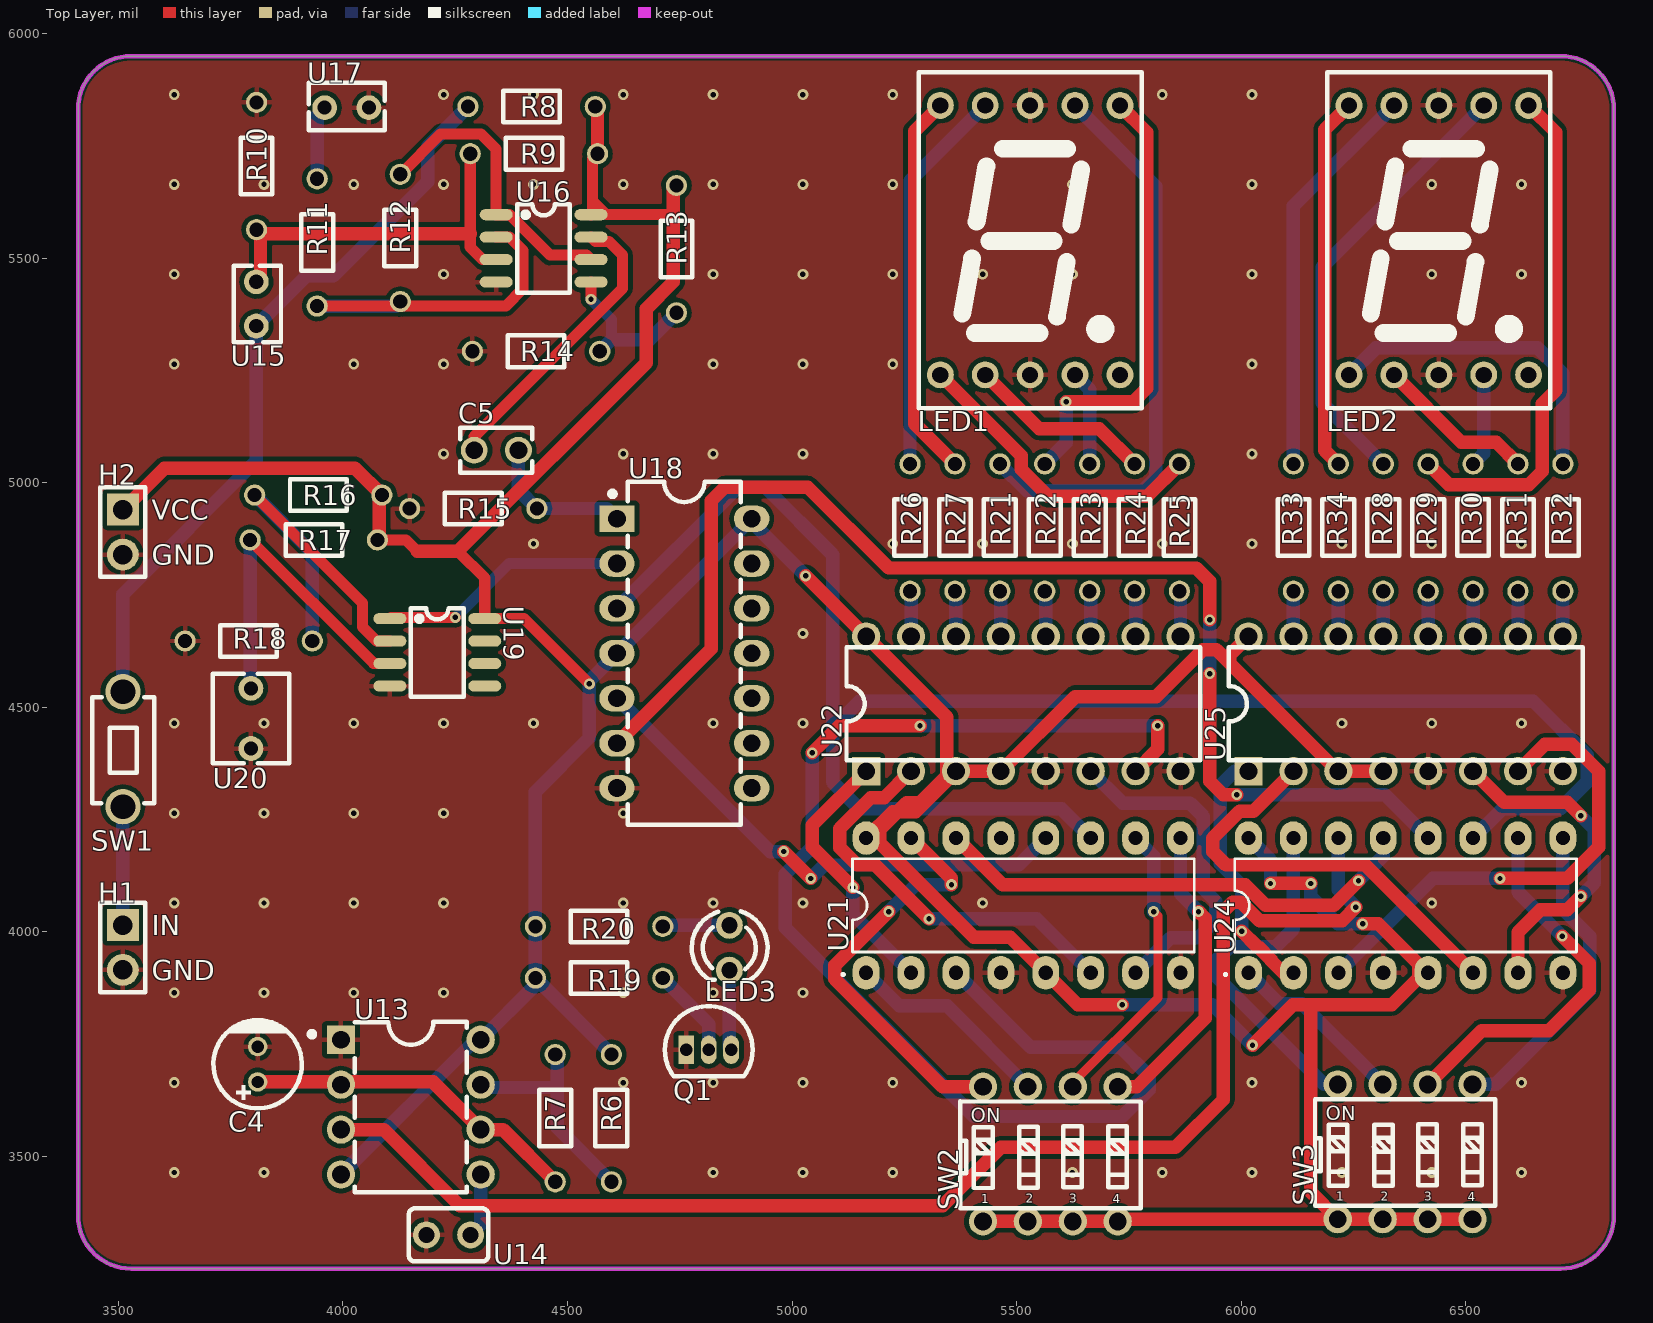
[diagram p0: Top Layer view]
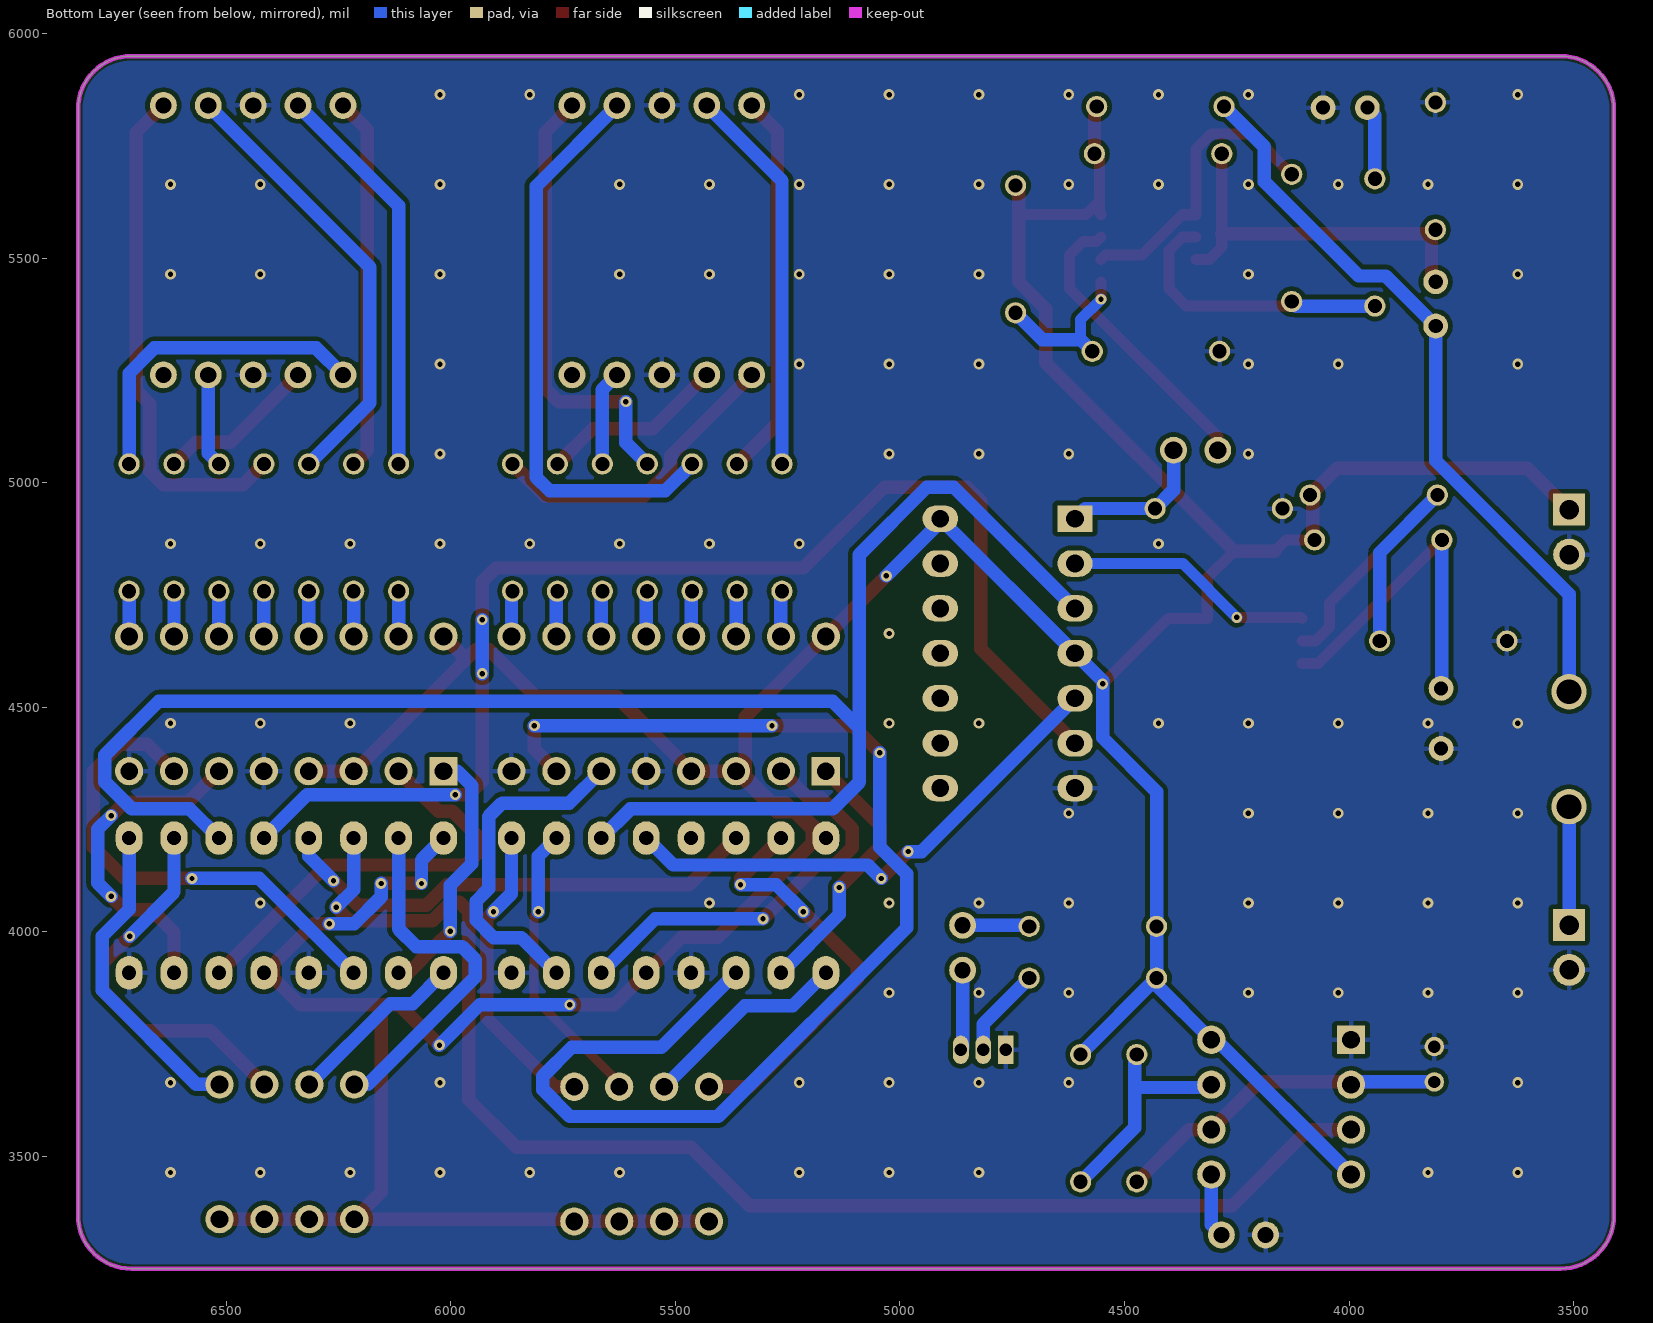
[diagram p1: Bottom Layer view, seen from below]
# Altium PCB MISC51104.pcbdoc
Units mil, origin at the board's own origin, x right, y up, seen from the top; angles counter-clockwise.
Board outline 3420 x 2700 mil, 2 copper layers (Top Layer, Bottom Layer), stack 62.206 mil thick; 52 components, 69 nets, 219 pads, 135 vias.

## Layer stack, top to bottom
Top Solder Mask Layer: solder mask 0.394, Dk 3.3
Top Layer: signal copper 1.379
Dielectric1: surface 59.449, FR4, Dk 4.5
Bottom Layer: signal copper 1.378
Bottom Solder Mask Layer: solder mask 0.394, Dk 3.3

## Board outline
3528.11,5950 ccw(c3528.11,5831.89) 3410,5831.89 3410,3368.11 ccw(c3528.11,3368.11) 3528.11,3250 6711.89,3250 ccw(c6711.89,3368.11) 6830,3368.11 6830,5831.89 ccw(c6711.89,5831.89) 6711.89,5950

## Design rules (kind name [scope] priority, off if disabled: settings)
BoardOutlineClearance copperThickness2oz_1 [All] p2 off: genericclearance=7.99 ignorepadtopadclearanceinfootprint=FALSE except(0: Arc-SplitContinuation Track-SplitContinuation SMDPad-SplitContinuation THPad-SplitContinuation Via-SplitContinuation Fill-SplitContinuation Region-SplitContinuation Poly-SplitContinuation Text-SplitContinuation Hole-SplitContinuation; 5.98: Arc-CutoutEdge Track-CutoutEdge SMDPad-CutoutEdge THPad-CutoutEdge Via-CutoutEdge Text-CutoutEdge; 6.89: Hole-OutlineEdge Hole-CutoutEdge; 10: Poly-OutlineEdge Poly-CutoutEdge; 11.81: Arc-OutlineEdge Track-OutlineEdge SMDPad-OutlineEdge THPad-OutlineEdge Via-OutlineEdge Fill-OutlineEdge Region-OutlineEdge Text-OutlineEdge Fill-CutoutEdge Region-CutoutEdge)
BoardOutlineClearance Plane_innerPlane_1 [All] p4 off: genericclearance=4.02 ignorepadtopadclearanceinfootprint=FALSE except(0: Arc-SplitContinuation Track-SplitContinuation SMDPad-SplitContinuation THPad-SplitContinuation Via-SplitContinuation Fill-SplitContinuation Region-SplitContinuation Poly-SplitContinuation Text-SplitContinuation Hole-SplitContinuation; 5.98: Arc-CutoutEdge Track-CutoutEdge SMDPad-CutoutEdge THPad-CutoutEdge Via-CutoutEdge Text-CutoutEdge; 6.89: Hole-OutlineEdge Hole-CutoutEdge; 10: Poly-OutlineEdge Poly-CutoutEdge; 11.81: Arc-OutlineEdge Track-OutlineEdge SMDPad-OutlineEdge THPad-OutlineEdge Via-OutlineEdge Fill-OutlineEdge Region-OutlineEdge Text-OutlineEdge Fill-CutoutEdge Region-CutoutEdge)
BoardOutlineClearance Copper_copperRegion_1 [All] p6 off: genericclearance=4.02 ignorepadtopadclearanceinfootprint=FALSE except(0: Arc-SplitContinuation Track-SplitContinuation SMDPad-SplitContinuation THPad-SplitContinuation Via-SplitContinuation Fill-SplitContinuation Region-SplitContinuation Poly-SplitContinuation Text-SplitContinuation Hole-SplitContinuation; 5.98: Arc-CutoutEdge Track-CutoutEdge SMDPad-CutoutEdge THPad-CutoutEdge Via-CutoutEdge Text-CutoutEdge; 6.89: Hole-OutlineEdge Hole-CutoutEdge; 10: Poly-OutlineEdge Poly-CutoutEdge; 11.81: Arc-OutlineEdge Track-OutlineEdge SMDPad-OutlineEdge THPad-OutlineEdge Via-OutlineEdge Fill-OutlineEdge Region-OutlineEdge Text-OutlineEdge Fill-CutoutEdge Region-CutoutEdge)
BoardOutlineClearance copperThickness1oz_1 [All] p8: genericclearance=4.02 ignorepadtopadclearanceinfootprint=FALSE except(0: Arc-SplitContinuation Track-SplitContinuation SMDPad-SplitContinuation THPad-SplitContinuation Via-SplitContinuation Fill-SplitContinuation Region-SplitContinuation Poly-SplitContinuation Text-SplitContinuation Hole-SplitContinuation; 5.98: Arc-CutoutEdge Track-CutoutEdge SMDPad-CutoutEdge THPad-CutoutEdge Via-CutoutEdge Text-CutoutEdge; 6.89: Hole-OutlineEdge Hole-CutoutEdge; 10: Poly-OutlineEdge Poly-CutoutEdge; 11.81: Arc-OutlineEdge Track-OutlineEdge SMDPad-OutlineEdge THPad-OutlineEdge Via-OutlineEdge Fill-OutlineEdge Region-OutlineEdge Text-OutlineEdge Fill-CutoutEdge Region-CutoutEdge)
Clearance copperThickness2oz [All] p1 off: gap=7.99 ignorepadtopadclearanceinfootprint=FALSE except(5.98: SMDPad-Track SMDPad-SMDPad THPad-Track SMDPad-THPad THPad-THPad Track-Via SMDPad-Via THPad-Via Via-Via Fill-SMDPad Region-SMDPad Fill-THPad Region-THPad Fill-Via Region-Via Fill-Fill Fill-Region Region-Region Arc-Track Arc-SMDPad Arc-THPad Arc-Via Fill-Arc Region-Arc Arc-Arc Text-Track SMDPad-Text Text-THPad Text-Via Fill-Text Region-Text Arc-Text Text-Text; 6.89: Hole-Track Hole-SMDPad Hole-THPad Hole-Via Fill-Hole Region-Hole Hole-Arc Hole-Text; 10: Poly-Track Poly-SMDPad Poly-THPad Poly-Via Poly-Fill Poly-Region Poly-Poly Poly-Arc Poly-Text Poly-Hole; 11.81: Fill-Track Region-Track)
Clearance Plane_innerPlane [All] p3 off: gap=4.02 ignorepadtopadclearanceinfootprint=FALSE except(5.98: SMDPad-Track SMDPad-SMDPad THPad-Track SMDPad-THPad THPad-THPad Track-Via SMDPad-Via THPad-Via Via-Via Fill-SMDPad Region-SMDPad Fill-THPad Region-THPad Fill-Via Region-Via Fill-Fill Fill-Region Region-Region Arc-Track Arc-SMDPad Arc-THPad Arc-Via Fill-Arc Region-Arc Arc-Arc Text-Track SMDPad-Text Text-THPad Text-Via Fill-Text Region-Text Arc-Text Text-Text; 6.89: Hole-Track Hole-SMDPad Hole-THPad Hole-Via Fill-Hole Region-Hole Hole-Arc Hole-Text; 10: Poly-Track Poly-SMDPad Poly-THPad Poly-Via Poly-Fill Poly-Region Poly-Poly Poly-Arc Poly-Text Poly-Hole; 11.81: Fill-Track Region-Track)
Clearance Copper_copperRegion [All] p5 off: gap=4.02 ignorepadtopadclearanceinfootprint=FALSE except(5.98: SMDPad-Track SMDPad-SMDPad THPad-Track SMDPad-THPad THPad-THPad Track-Via SMDPad-Via THPad-Via Via-Via Fill-SMDPad Region-SMDPad Fill-THPad Region-THPad Fill-Via Region-Via Fill-Fill Fill-Region Region-Region Arc-Track Arc-SMDPad Arc-THPad Arc-Via Fill-Arc Region-Arc Arc-Arc Text-Track SMDPad-Text Text-THPad Text-Via Fill-Text Region-Text Arc-Text Text-Text; 6.89: Hole-Track Hole-SMDPad Hole-THPad Hole-Via Fill-Hole Region-Hole Hole-Arc Hole-Text; 10: Poly-Track Poly-SMDPad Poly-THPad Poly-Via Poly-Fill Poly-Region Poly-Poly Poly-Arc Poly-Text Poly-Hole; 11.81: Fill-Track Region-Track)
Clearance copperThickness1oz [All] p7: gap=4.02 ignorepadtopadclearanceinfootprint=FALSE except(5.98: SMDPad-Track SMDPad-SMDPad THPad-Track SMDPad-THPad THPad-THPad Track-Via SMDPad-Via THPad-Via Via-Via Fill-SMDPad Region-SMDPad Fill-THPad Region-THPad Fill-Via Region-Via Fill-Fill Fill-Region Region-Region Arc-Track Arc-SMDPad Arc-THPad Arc-Via Fill-Arc Region-Arc Arc-Arc Text-Track SMDPad-Text Text-THPad Text-Via Fill-Text Region-Text Arc-Text Text-Text; 6.89: Hole-Track Hole-SMDPad Hole-THPad Hole-Via Fill-Hole Region-Hole Hole-Arc Hole-Text; 10: Poly-Track Poly-SMDPad Poly-THPad Poly-Via Poly-Fill Poly-Region Poly-Poly Poly-Arc Poly-Text Poly-Hole; 11.81: Fill-Track Region-Track)
DiffPairsRouting differentialPair [All] p1: maxlimit=6 minlimit=6 mostfreqgap=6 toplayer_minwidth=5 toplayer_prefwidth=10 toplayer_maxwidth=100 toplayer_mingap=6 toplayer_prefgap=6 toplayer_maxgap=6 bottomlayer_minwidth=5 bottomlayer_prefwidth=10 bottomlayer_maxwidth=100 bottomlayer_mingap=6 bottomlayer_prefgap=6 bottomlayer_maxgap=6 maxuncoupledlength=10
HoleToHoleClearance otherClearance [All] p1: gap=11.81 allowstackedmicrovias=TRUE
Length netLength [All] p1: minlimit=0 maxlimit=0
PasteMaskExpansion pasteMaskExpansion [All] p1: expansion=0
PlaneConnect innerPlane [All] p1: planeconnectstyle=Relief reliefexpansion=20 reliefentries=4 reliefconductorwidth=10 reliefairgap=10
PolygonConnect copperRegion [All] p1: connectstyle=Relief reliefconductorwidth=10 reliefentries=4 polygonreliefangle="90 Angle" airgapwidth=10 via.connectstyle=Relief via.reliefconductorwidth=10 via.reliefentries=4 via.polygonreliefangle="90 Angle" via.airgapwidth=10
RoutingVias viaSize [All] p1: holewidth=12.01 width=24.02 viastyle="Through Hole" minholewidth=11.81 minwidth=19.68 maxholewidth=248.03 maxwidth=393.7
SolderMaskExpansion solderMaskExpansion [IsVia] p1: expansion=-1000 istentingtop=TRUE
SolderMaskExpansion solderMaskExpansion [All] p2: expansion=2.01 istentingtop=FALSE
Width copperThickness2oz_2 [All] p1 off: maxlimit=100 minlimit=8 preferedwidth=10
Width copperThickness1oz_2 [All] p2: maxlimit=100 minlimit=5 preferedwidth=30

## Components (designator, comment, footprint, x,y, rotation, side; value= is the part's Value field where it differs from the comment)
C4 "10uF" CAP-TH_BD5.0-P2.00-D0.5-FD 3810,3705 r90 top
C5 "100nF" CAP-TH_L4.0-W2.5-P2.50-D0.5-A 4341.4,5072.26 r0 top
H1 "" HDR-TH_2P-P2.54-V-M-1 3510,3965 r270 top
H2 "" HDR-TH_2P-P2.54-V-M-1 3510,4890 r270 top
LED1 "" LED-SEG-TH_10P-L12.6-W19.0-P2.54-S15.24-BL 5530,5540 r0 top
LED2 "" LED-SEG-TH_10P-L12.6-W19.0-P2.54-S15.24-BL 6440,5540 r0 top
LED3 "" LED_TH-3mm 4860.3,3964.43 r270 top
Q1 "2N2222A" TO-92-3_L4.9-W3.7-P1.27-L 4814.38,3737.18 r0 top
R6 "47kΩ" Res_1/8W 4600,3585 r90 top
R7 "47kΩ" Res_1/8W 4475,3585 r90 top
R8 "4.7kΩ" Res_1/8W 4420,5835 r0 top
R9 "4.7kΩ" Res_1/8W 4425,5730 r0 top
R10 "4.7kΩ" Res_1/8W 3805,5705 r270 top
R11 "1kΩ" Res_1/8W 3940,5535 r270 top
R12 "100kΩ" Res_1/8W 4130,5545 r90 top
R13 "10kΩ" Res_1/8W 4745,5520 r90 top
R14 "2kΩ" Res_1/8W 4430,5290 r0 top
R15 "10kΩ" Res_1/8W 4290,4940 r0 top
R16 "100kΩ" Res_1/8W 3945,4970 r0 top
R17 "100kΩ" Res_1/8W 3935,4870 r0 top
R18 "100kΩ" Res_1/8W 3790,4645 r0 top
R19 "3kΩ" Res_1/8W 4570.3,3899.43 r180 top
R20 "200Ω" Res_1/8W 4570.3,4014.43 r180 top
R21 "10kΩ" Res_1/8W 5465,4900 r90 top
R22 "10kΩ" Res_1/8W 5565,4900 r90 top
R23 "10kΩ" Res_1/8W 5665,4900 r90 top
R24 "10kΩ" Res_1/8W 5765,4900 r90 top
R25 "10kΩ" Res_1/8W 5865,4900 r90 top
R26 "10kΩ" Res_1/8W 5265,4900 r90 top
R27 "10kΩ" Res_1/8W 5365,4900 r90 top
R28 "10kΩ" Res_1/8W 6318.74,4900 r90 top
R29 "10kΩ" Res_1/8W 6418.74,4900 r90 top
R30 "10kΩ" Res_1/8W 6518.74,4900 r90 top
R31 "10kΩ" Res_1/8W 6618.74,4900 r90 top
R32 "10kΩ" Res_1/8W 6718.74,4900 r90 top
R33 "10kΩ" Res_1/8W 6118.74,4900 r90 top
R34 "10kΩ" Res_1/8W 6218.74,4900 r90 top
SW1 "" Key_TH_3.5x6x4.3 3510,4400 r90 top
SW2 "拨码开关EI-04" SW-TH_DIPSWITCHEI-04 5575,3505 r0 top
SW3 "拨码开关EI-04" SW-TH_DIPSWITCHEI-04 6365,3510 r0 top
U13 "NE555PE4" PDIP-8_L9.6-W6.4-P2.54-LS7.9-BL-1 4151.02,3609.58 r270 top
U14 "100nF" CAP-TH_L4.5-W3.0-P2.50-D0.5 4235,3325 r0 top
U15 "1uF" CAP-TH_L4.0-W2.5-P2.50-D0.5 3806.97,5398.05 r90 top
U16 "LM358AD" SOP-8_L4.9-W3.9-P1.27-LS6.0-BL 4446.68,5521.68 r270 top
U17 "1uF" CAP-TH_L4.0-W2.5-P2.50-D0.5 4008.42,5835 r180 top
U18 "CD4011BD" PDIP-14_L19.3-W6.4-P2.54-LS7.9-BL-1 4760,4620 r270 top
U19 "LM358AD" SOP-8_L4.9-W3.9-P1.27-LS6.0-BL 4210.07,4622.26 r270 top
U20 "光敏电阻-5MM" RES-TH_L4.9-W4.3-P3.4 3795,4475 r90 top
U21 "SN74LS190N" PDIP-16_L19.2-W6.6-P2.54-LS7.6-BL 5514.82,4058.71 r0 top
U22 "CD4511BE" DIP-16_L19.8-W6.5-P2.54-LS7.6-BL 5514.82,4507.64 r0 top
U24 "SN74LS190N" PDIP-16_L19.2-W6.6-P2.54-LS7.6-BL 6366.27,4058.71 r0 top
U25 "CD4511BE" DIP-16_L19.8-W6.5-P2.54-LS7.6-BL 6366.27,4507.64 r0 top

## Footprints (in the part's own frame and the unit in brackets; to place one, negate y for a bottom-side part, rotate by r counter-clockwise, add the part's x,y. Pads: shape width x height; smd on the part's side, far side on the other; paste and mask are expansions set on the pad)
CAP-TH_BD5.0-P2.00-D0.5-FD [mm]
  round 1.1 hole 0.7 paste+0 mask+0.05: 1(-1,0) 2(1,0)
  silkscreen extent -2.5,-2.5 2.5,2.5
CAP-TH_L4.0-W2.5-P2.50-D0.5 [mm]
  round 1.4 hole 0.8 paste+0 mask+0.05: 1(-1.25,0) 2(1.25,0)
  silkscreen extent -2.16,-1.4 2.16,1.27
CAP-TH_L4.0-W2.5-P2.50-D0.5-A [mil]
  round 60 hole 39.37 paste+0 mask+1.97: 1(-49.21,0) 2(49.21,0)
  silkscreen extent -80,-50 80,50
CAP-TH_L4.5-W3.0-P2.50-D0.5 [mil]
  round 60 hole 36 paste+0 mask+1.97: 1(-49.21,0) 2(49.21,0)
  silkscreen extent -89,-59 89,59
DIP-16_L19.8-W6.5-P2.54-LS7.6-BL [mm]
  rect 1.6x1.6 hole 1: 1(-8.89,-3.81)
  round 1.6 hole 1 copper offset 0,0: 2(-6.35,-3.81) 3(-3.81,-3.81) 4(-1.27,-3.81) 5(1.27,-3.81) 6(3.81,-3.81) 7(6.35,-3.81) 8(8.89,-3.81) 9(8.89,3.81) 10(6.35,3.81) 11(3.81,3.81) 12(1.27,3.81) 13(-1.27,3.81) 14(-3.81,3.81) 15(-6.35,3.81) 16(-8.89,3.81)
  silkscreen extent -10,-3.2 10,3.2
HDR-TH_2P-P2.54-V-M-1 [mm]
  rect 1.8x1.8 hole 1.1: 1(-1.27,0)
  round 1.8 hole 1.1: 2(1.27,0)
  silkscreen extent -2.54,-1.27 2.54,1.27
Key_TH_3.5x6x4.3 [mil]
  round 78.7 hole 55.1 paste+0 mask+2: A(-121.44,0) B(134.46,0)
  silkscreen extent -114,-70 123,68
LED-SEG-TH_10P-L12.6-W19.0-P2.54-S15.24-BL [mil]
  round 60 hole 36: 1(-200,-300) 2(-100,-300) 3(0,-300) 4(100,-300) 5(200,-300) 6(200,300) 7(100,300) 8(0,300) 9(-100,300) 10(-200,300)
  silkscreen extent -248,-374 248,374
LED_TH-3mm [mil]
  round 60 hole 36 paste+0 mask+2: 1(-50,0) 2(50,0)
  silkscreen extent -81,-84 72,85
PDIP-8_L9.6-W6.4-P2.54-LS7.9-BL-1 [mil]
  rect 63x63 hole 39.37: 1(-150,-155.51)
  round 63 hole 39.37: 2(-50,-155.51) 3(50,-155.51) 4(150,-155.51) 5(150,155.52) 6(50,155.52) 7(-50,155.52) 8(-150,155.52)
  silkscreen extent -190,-226 190,125
PDIP-14_L19.3-W6.4-P2.54-LS7.9-BL-1 [mm]
  rect 1.5x2 hole 1: 1(-7.62,-3.81)
  oval 1.5x2 hole 1: 2(-5.08,-3.81) 3(-2.54,-3.81) 4(0,-3.81) 5(2.54,-3.81) 6(5.08,-3.81) 7(7.62,-3.81)
  oval 1.5x2 hole 1 copper offset 0,0: 8(7.62,3.81) 9(5.08,3.81) 10(2.54,3.81) 11(0,3.81) 12(-2.54,3.81) 13(-5.08,3.81) 14(-7.62,3.81)
  silkscreen extent -9.7,-4.21 9.7,3.2
PDIP-16_L19.2-W6.6-P2.54-LS7.6-BL [mm]
  oval 1.52x1.9 hole 0.8: 1(-8.89,-3.81) 2(-6.35,-3.81) 3(-3.81,-3.81) 4(-1.27,-3.81) 5(1.27,-3.81) 6(3.81,-3.81) 7(6.35,-3.81) 8(8.89,-3.81) 9(8.89,3.81) 10(6.35,3.81) 11(3.81,3.81) 12(1.27,3.81) 13(-1.27,3.81) 14(-3.81,3.81) 15(-6.35,3.81) 16(-8.89,3.81)
  silkscreen extent -10.26,-3.98 9.66,2.63
RES-TH_L4.9-W4.3-P3.4 [mm]
  round 1.4 hole 0.8 paste+0 mask+0.05: 1(-1.7,0) 2(1.7,0)
  silkscreen extent -2.54,-2.16 2.54,2.16
Res_1/8W [mil]
  round 47.2 hole 31.5 paste+0 mask+2: 1(-141.7,2.48) 2(141.7,2.48)
  silkscreen extent -63,-33 63,38
SOP-8_L4.9-W3.9-P1.27-LS6.0-BL [mm]
  oval 0.63x1.865 smd: 1(-1.905,-2.682) 2(-0.635,-2.682) 3(0.635,-2.682) 4(1.905,-2.682) 5(1.905,2.682) 6(0.635,2.682) 7(-0.635,2.682) 8(-1.905,2.682)
  silkscreen extent -2.5,-1.5 2.5,1.48
SW-TH_DIPSWITCHEI-04 [mm]
  round 1.6 hole 1: 1(-3.81,-3.81) 2(-1.27,-3.81) 3(1.27,-3.81) 4(3.81,-3.81) 5(3.81,3.81) 6(1.27,3.81) 7(-1.27,3.81) 8(-3.81,3.81)
  silkscreen extent -5.1,-3.05 5.11,2.98
TO-92-3_L4.9-W3.7-P1.27-L [mm]
  rect 0.9x1.6 hole 0.7: 1(-1.27,0)
  oval 0.9x1.6 hole 0.7: 2(0,0) 3(1.27,0)
  silkscreen extent -2.48,-1.5 2.48,2.48

## Via types
v1: diameter 24.02, hole 12, Top Layer to Bottom Layer, 134 vias
v2: diameter 24, hole 12, Top Layer to Bottom Layer, 1 vias

## Nets (pads, with @x,y where several pads share a name; then routed paths per layer and width w, separated by ;. In a path a pad name is that pad's centre, name@x,y a point inside that pad or via, vN(x,y) a via of type N, cw(c..) or ccw(c..) an arc to the next point about the centre after c; other vN are vias at no path point)
$1N1893: R6.1 R7.2 U13.7 | length 508.8
  Bottom Layer w30: U13.7 4312.81,3653.3 4477.52,3653.3 ; R7.2 4477.52,3721.7 4477.52,3653.3 ; R6.1 4477.52,3563.3 4477.52,3653.3
$1N1894: C4.1 R7.1 U13.2 U13.6 | length 942.6
  Top Layer w30: C4.1 4200.48,3665.63 U13.6 4356.25,3559.58 R7.1
  Bottom Layer w30: C4.1 3989.46,3665.63 U13.2
$1N1895: U13.5 U14.2 | length 143.8
  Bottom Layer w30: U14.2 4306.53,3347.32 U13.5
$1N1964: H1.1 SW1.A | length 263.6
  Bottom Layer w30: H1.1 SW1.A
$1N2089: R8.1 SW1.B U15.1 | length 1656.4
  Bottom Layer w30: SW1.B 3510,4751.87 3806.97,5048.84 U15.1 3918.3,5460.17 3978.3,5460.17 4188.3,5670.17 4188.3,5747.48 R8.1
$1N2753: R9.1 R10.2 U15.2 U16.3 | length 867.9
  Top Layer w24.8: R9.1 4283.3,5554.44 4283.3,5524.44 4311.07,5496.68 U16.3
  Top Layer w30: U15.2 3816.33,5456.63 R10.2@3816.33,5554.44 ; R10.2 R10.2@3816.33,5554.44 ; 4283.3,5554.44 R10.2@3816.33,5554.44
$1N2866: R11.1 U17.2 | length 165.2
  Bottom Layer w30: R11.1 3942.48,5818.27 U17.2
$1N2941: R12.2 U16.1 U16.6 | length 663.8
  Top Layer w24.8: R12.2 4217.52,5776.7 4307.52,5776.7 4341.07,5743.16 U16.1 4371.07,5596.68 4461.07,5506.68 4542.29,5506.68 U16.6
$1N2947: R11.2 R12.1 U16.2 | length 821
  Top Layer w24.8: R11.2 4362.48,5393.3 4401.07,5431.89 4401.07,5516.68 4371.07,5546.68 U16.2
  Bottom Layer w30: R11.2 4117.52,5393.3 R12.1
$1N3011: R13.1 R14.2 U16.5 | length 353.5
  Top Layer w24.8: v1(4552.29,5408.3) U16.5
  Bottom Layer w24.8: v1(4552.29,5408.3) 4597.52,5363.06 4597.52,5318.3
  Bottom Layer w30: R14.2 4597.52,5318.3 4682.52,5318.3 R13.1
$1N3176: C5.1 U16.7 | length 657.6
  Top Layer w24.8: C5.1 4292.19,5102.26 4622.19,5432.26 4622.19,5506.77 4592.19,5536.77 4562.19,5536.77 U16.7
$1N3286: C5.2 R15.2 U18.1 | length 334.4
  Bottom Layer w30: C5.2 4390.61,4983.56 R15.2 4587.53,4942.48 U18.1
$1N6918: U18.2 U19.1 | length 556.4
  Top Layer w24.8: U19.1 4107.2,4700 v1(4250,4700)
  Bottom Layer w24.8: v1(4250,4700) 4370,4820 U18.2
$1N7003: R17.1 U19.3 U20.2 | length 756.4
  Top Layer w24.8: R17.1 4068.52,4597.26 U19.3
  Bottom Layer w30: R17.1 3793.3,4543.63 U20.2
$1N7096: R16.1 R18.2 U19.2 | length 845.7
  Top Layer w24.8: R16.1 4043.3,4732.48 4043.3,4678.42 4074.46,4647.26 U19.2
  Bottom Layer w30: R16.1 3931.7,4844.08 R18.2
$1N10184: R26.1 U22.15 | length 101.6
  Bottom Layer w30: R26.1 5264.82,4756.01 U22.15
$1N10187: LED1.9 R26.2 | length 867.7
  Bottom Layer w30: R26.2 5262.52,5672.52 LED1.9
$1N10190: R27.1 U22.14 | length 101.6
  Bottom Layer w30: R27.1 5364.82,4756.01 U22.14
$1N10193: LED1.10 R27.2 | length 859.4
  Top Layer w30: LED1.10 5272.52,5782.52 5272.52,5131.7 R27.2
$1N10196: R21.1 U22.13 | length 101.6
  Bottom Layer w30: R21.1 5464.82,4756.01 U22.13
$1N10199: LED1.7 R21.2 | length 1287.6
  Bottom Layer w30: R21.2 5522.52,4981.7 5780,4981.7 5810,5011.7 5810,5660 LED1.7
$1N10202: R22.1 U22.12 | length 101.6
  Bottom Layer w30: R22.1 5564.82,4756.01 U22.12
$1N10205: LED1.6 R22.2 | length 1005.2
  Top Layer w30: v1(5610,5180) 5760,5180 5790,5210 5790,5780 LED1.6
  Bottom Layer w30: R22.2 5610,5089.18 v1(5610,5180)
$1N10208: R23.1 U22.11 | length 101.6
  Bottom Layer w30: R23.1 5664.82,4756.01 U22.11
$1N10211: LED1.4 R23.2 | length 211.8
  Bottom Layer w30: LED1.4 5662.52,5207.48 R23.2
$1N10214: R24.1 U22.10 | length 101.6
  Bottom Layer w30: R24.1 5764.82,4756.01 U22.10
$1N10217: LED1.2 R24.2 | length 414.7
  Top Layer w30: LED1.2 5550,5120 5684.22,5120 R24.2
$1N10220: R25.1 U22.9 | length 101.6
  Bottom Layer w30: R25.1 5864.82,4756.01 U22.9
$1N10223: LED1.1 R25.2 | length 691.6
  Top Layer w30: LED1.1 5510,5060 5510,5030 5570,4970 5790.82,4970 R25.2
$1N10225: U21.2 U22.1 | length 589.8
  Top Layer w30: v1(5134.82,4098.71) 5044.82,4188.71 5044.82,4237.64 U22.1
  Bottom Layer w30: v1(5134.82,4098.71) 5134.82,4038.71 U21.2
$1N10227: U21.3 U22.7 | length 2894.1
  Top Layer w30: v1(5044.82,4398.71) 5104.82,4458.71 v1(5284.82,4458.71) ; U22.7 5813.75,4406.57 v1(5813.75,4458.71)
  Bottom Layer w30: v1(5044.82,4398.71) 5044.82,4188.71 4984.82,4128.71 4984.82,4008.71 5404.82,3588.71 5734.82,3588.71 5794.82,3648.71 5794.82,3678.71 5730.88,3742.64 5530.88,3742.64 U21.3 ; v1(5284.82,4458.71) v1(5813.75,4458.71)
$1N10229: U21.6 U22.2 | length 928.4
  Top Layer w30: U22.2 5263.75,4357.64 5204.82,4298.71 5174.82,4298.71 5106.03,4229.92 5106.03,4187.49 5144.82,4148.71 5184.82,4148.71 v1(5304.82,4028.71)
  Bottom Layer w30: v1(5304.82,4028.71) 5544.82,4028.71 U21.6
$1N10231: U21.7 U22.6 | length 762.7
  Bottom Layer w30: U22.6 5735.89,4286.57 5885.89,4286.57 5915.89,4256.57 5915.89,4095.5 5943.6,4067.78 5943.6,4025.35 5904.82,3986.57 5842.68,3986.57 U21.7
$1N10411: SW2.7 U21.1 | length 465.3
  Bottom Layer w30: U21.1 5238.52,3835 5345,3835 SW2.7
$1N10413: SW2.5 U21.9 | length 682.2
  Top Layer w30: SW2.5 5767.43,3655 5920,3807.57 5920,4030 v1(5905,4045)
  Bottom Layer w30: U21.9 5864.82,4085.18 v1(5905,4045)
$1N10415: SW2.6 U21.10 | length 653.2
  Top Layer w20: SW2.6 5625,3663.31 5815,3853.31 5815,4035 v1(5805,4045)
  Bottom Layer w30: U21.10 5805,4168.52 v1(5805,4045)
$1N10417: SW2.8 U21.15 | length 934.8
  Top Layer w30: v1(5215,4045) 5095,3925 5095,3895 5335,3655 SW2.8 ; U21.15 5354.82,4118.71 v1(5354.82,4105)
  Bottom Layer w30: v1(5215,4045) 5275,4105 v1(5354.82,4105)
$1N10829: U24.2 U25.1 | length 575.2
  Top Layer w30: v1(6001.27,4001.11) 6035.28,3967.09 6037.35,3967.09 6067.17,3937.27 6067.17,3935.2 6093.67,3908.71 U24.2
  Bottom Layer w30: v1(6001.27,4001.11) 6001.27,4103.71 5953.23,4151.74 5953.23,4325.67 5985.2,4357.64 U25.1
$1N10831: U24.6 U25.2 | length 963.5
  Top Layer w30: U25.2 6027.34,4268.71 5996.27,4268.71 5936.27,4208.71 5936.27,4178.71 5966.27,4148.71 6276.27,4148.71 U24.6
$1N10833: U24.7 U25.6 | length 749
  Top Layer w30: U25.6 6585.2,4288.71 6726.27,4288.71 v1(6756.27,4258.71) ; U24.7 6616.27,3998.71 6666.27,4048.71 6726.27,4048.71 v1(6756.27,4078.71)
  Bottom Layer w30: v1(6756.27,4078.71) 6786.27,4108.71 6786.27,4228.71 v1(6756.27,4258.71)
$1N10844: SW3.5 U24.9 | length 711.8
  Bottom Layer w30: SW3.5 6566.27,3660 6776.27,3870 6776.27,3990 6716.27,4050 U24.9
$1N10846: SW3.7 U24.1 | length 401.8
  Bottom Layer w30: U24.1 6084.97,3840 6135,3840 SW3.7
$1N10848: SW3.6 U24.10 | length 851.4
  Top Layer w30: SW3.6 6535,3780 6685,3780 6775,3870 6775,3930 v1(6715,3990)
  Bottom Layer w30: U24.10 6616.27,4088.73 v1(6715,3990)
$1N10850: LED2.6 R29.2 | length 1137.2
  Top Layer w30: R29.2 6462.53,4995.43 6640,4995.43 6670,5025.43 6670,5175.43 6700,5205.43 6700,5780 LED2.6
$1N10852: LED2.4 R30.2 | length 208.1
  Bottom Layer w30: R30.2 6540,5065.43 LED2.4
$1N10854: LED2.2 R31.2 | length 358.4
  Top Layer w30: LED2.2 6490,5090 6567.97,5090 R31.2
$1N10856: LED2.1 R32.2 | length 726.5
  Bottom Layer w30: LED2.1 6300,5300 6660,5300 6716.27,5243.73 R32.2
$1N10858: LED2.9 R33.2 | length 891
  Bottom Layer w30: R33.2 6116.27,5616.27 LED2.9
$1N10860: LED2.10 R34.2 | length 833
  Top Layer w30: R34.2 6186.27,5071.7 6186.27,5786.27 LED2.10
$1N10862: R33.1 U25.15 | length 100.7
  Bottom Layer w30: U25.15 R33.1
$1N10864: R34.1 U25.14 | length 100.7
  Bottom Layer w30: U25.14 R34.1
$1N10866: R29.1 U25.12 | length 100.7
  Bottom Layer w30: U25.12 R29.1
$1N10868: R30.1 U25.11 | length 100.7
  Bottom Layer w30: U25.11 R30.1
$1N10870: R31.1 U25.10 | length 100.7
  Bottom Layer w30: U25.10 R31.1
$1N10872: R32.1 U25.9 | length 100.7
  Bottom Layer w30: U25.9 R32.1
$1N10874: SW3.8 U24.15 | length 808.9
  Bottom Layer w30: U24.15 6116.27,4006.27 6077.09,3967.09 5975,3967.09 5945,3937.09 5945,3900 6185,3660 SW3.8
$1N10876: U24.3 U25.7 | length 1094.6
  Top Layer w30: v1(6576.27,4118.71) 6726.27,4118.71 6796.27,4188.71 6796.27,4357.64 6736.27,4417.64 6676.27,4417.64 U25.7
  Bottom Layer w30: U24.3 6426.27,4118.71 v1(6576.27,4118.71)
$1N10878: R28.1 U25.13 | length 100.7
  Bottom Layer w30: U25.13 R28.1
$1N10880: LED2.7 R28.2 | length 1003.9
  Bottom Layer w30: R28.2 6180,5177.97 6180,5480 LED2.7
$1N10977: U18.3 U21.11 U24.11 | length 3907
  Bottom Layer w30: U18.3 4880,4990 4940,4990 5090,4840 5090,4453.52 ; U21.11 5600,4273.52 5150,4273.52 5090,4333.52 5090,4453.52 ; U24.11 6581.08,4273.52 6710,4273.52 6770,4333.52 6770,4393.52 6650,4513.52 5150,4513.52 5090,4453.52
$1N10992: U21.14 U24.13 | length 1099.1
  Top Layer w30: U21.14 5468.52,4105 6008.52,4105 6054.82,4058.71 6206.27,4058.71 v1(6261.27,4113.71)
  Bottom Layer w30: v1(6261.27,4113.71) 6316.27,4168.71 U24.13
$1N11009: U18.5 U21.12 | length 1158.3
  Top Layer w30: v1(4981.29,4178.71) v1(5041.29,4118.71)
  Bottom Layer w30: U18.5 4951.29,4178.71 v1(4981.29,4178.71) ; v1(5041.29,4118.71) 5071.29,4148.71 5504.82,4148.71 U21.12
$1N11018: U18.6 U24.12 | length 2820
  Top Layer w30: U18.6 4820,4630 4820,4960 4850,4990 5035,4990 5215,4810 5900,4810 5930,4780 v1(5930,4694.97) ; v1(5930,4574.97) 5930,4334.97 5960,4304.97 v1(5990,4304.97)
  Bottom Layer w30: v1(5930,4574.97) v1(5930,4694.97) ; v1(5990,4304.97) 6320,4304.97 U24.12
$1N11115: U13.3 U24.14 | length 3054.6
  Top Layer w30: U13.3 4090.42,3559.58 4260,3390 5335,3390 5465,3520 5853.69,3520 5960,3626.31 5960,4045 5981.21,4066.21 5999.2,4066.21 6040.73,4024.69 6224.69,4024.69 v2(6255,4055)
  Bottom Layer w30: U24.14 6216.27,4093.73 v2(6255,4055)
$1N11198: Q1.2 R19.1 | length 202.2
  Bottom Layer w30: R19.1 4814.38,3794.58 Q1.2
$1N11296: LED3.2 Q1.3 | length 178.9
  Bottom Layer w30: LED3.2 4860.3,3741.25 Q1.3
$1N11369: LED3.1 R20.1 | length 149.3
  Bottom Layer w30: R20.1 4714.48,4014.43 LED3.1
GND: C4.2 H1.2 H2.2 LED1.3 LED1.8 LED2.3 LED2.8 Q1.1 R10.1 R14.1 R15.1 R18.1 U13.1 U14.1 U16.4 U17.1 U18.7 U19.4 U20.1 U21.4 U21.8 U22.5 U22.8 U24.4 U24.8 U25.5 U25.8
  other v1: 3624.1,3464.1 3824.1,3464.1 4824.1,3464.1 5024.1,3464.1 5224.1,3464.1 5624.1,3464.1 5824.1,3464.1 6024.1,3464.1 6224.1,3464.1 6424.1,3464.1 6624.1,3464.1 3624.1,3664.1 4624.1,3664.1 4824.1,3664.1 5024.1,3664.1 5224.1,3664.1 6024.1,3664.1 6624.1,3664.1 3624.1,3864.1 3824.1,3864.1 4024.1,3864.1 4224.1,3864.1 4624.1,3864.1 4824.1,3864.1 5024.1,3864.1 3624.1,4064.1 3824.1,4064.1 4024.1,4064.1 4224.1,4064.1 4624.1,4064.1 4824.1,4064.1 5024.1,4064.1 5424.1,4064.1 6424.1,4064.1 3624.1,4264.1 3824.1,4264.1 4024.1,4264.1 4224.1,4264.1 4624.1,4264.1 3624.1,4464.1 3824.1,4464.1 4024.1,4464.1 4224.1,4464.1 4424.1,4464.1 4824.1,4464.1 5024.1,4464.1 6224.1,4464.1 6424.1,4464.1 6624.1,4464.1 5024.1,4664.1 4424.1,4864.1 5224.1,4864.1 5424.1,4864.1 5624.1,4864.1 5824.1,4864.1 6024.1,4864.1 6224.1,4864.1 6424.1,4864.1 6624.1,4864.1 4224.1,5064.1 4624.1,5064.1 4824.1,5064.1 5024.1,5064.1 6024.1,5064.1 3624.1,5264.1 4024.1,5264.1 4224.1,5264.1 4824.1,5264.1 5024.1,5264.1 5224.1,5264.1 6024.1,5264.1 3624.1,5464.1 4224.1,5464.1 4824.1,5464.1 5024.1,5464.1 5224.1,5464.1 5424.1,5464.1 5624.1,5464.1 6024.1,5464.1 6424.1,5464.1 6624.1,5464.1 3624.1,5664.1 3824.1,5664.1 4024.1,5664.1 4224.1,5664.1 4424.1,5664.1 4624.1,5664.1 4824.1,5664.1 5024.1,5664.1 5224.1,5664.1 5424.1,5664.1 5624.1,5664.1 6024.1,5664.1 6424.1,5664.1 6624.1,5664.1 3624.1,5864.1 4224.1,5864.1 4424.1,5864.1 4624.1,5864.1 4824.1,5864.1 5024.1,5864.1 5224.1,5864.1 5824.1,5864.1 6024.1,5864.1
VCC: H2.1 R6.2 R8.2 R9.2 R13.2 R16.2 R17.2 R19.2 R20.2 SW2.1 SW2.2 SW2.3 SW2.4 SW3.1 SW3.2 SW3.3 SW3.4 U13.4 U13.8 U16.8 U18.4 U18.14 U19.8 U21.5 U21.16 U22.3 U22.4 U22.16 U24.5 U24.16 U25.3 U25.4 U25.16 | length 11110
  Top Layer w24.8: R17.2 4080.46,4872.48 4140.46,4872.48 4165.68,4847.26 ; 4255.68,4847.26 4315.68,4787.26 U19.8 4403.3,4697.26 v1(4548.6,4551.96) ; U16.8 4555.68,5600.07 4555.68,5627.26 ; R9.2 4555.68,5721.46 4555.68,5627.26 ; 4735.68,5597.26 4585.68,5597.26 4555.68,5627.26
  Top Layer w30: H2.1 3602.48,5032.48 4026.7,5032.48 R16.2 4080.46,4966.24 R17.2@4080.46,4872.48 ; 4165.68,4847.26 4255.68,4847.26 4675.68,5267.26 4675.68,5387.26 4735.68,5447.26 4735.68,5597.26 4735.68,5654.86 R13.2 ; R8.2 4566.7,5832.48 R9.2 ; v1(5030,4792.45) U22.16 5344.82,4477.64 U22.3@5344.82,4377.64 ; U21.16 5223.75,4267.64 5234.82,4267.64 ; SW2.1 SW2.2 SW2.3 SW2.4 5730,3360 SW3.1 ; v1(5735.2,3837.64) 5635.89,3837.64 U21.5 5485.89,3987.64 5404.82,3987.64 5194.82,4197.64 5194.82,4227.64 5234.82,4267.64 ; U25.16 5974.82,4616.19 5974.82,4597.64 ; v1(6025.2,3747.64) 6115.2,3837.64 6155.2,3837.64 ; v1(6065.2,4107.64) v1(6155.2,4107.64) ; v1(6270.2,4017.64) 6305.2,4017.64 6395.2,3927.64 U24.5@6395.2,3897.64 ; U25.4 U25.3 6214.82,4357.64 5974.82,4597.64 ; U24.5 6405.2,3897.64 U24.5@6395.2,3897.64 ; SW3.4 SW3.3 SW3.2 SW3.1 ; 5234.82,4267.64 5274.82,4267.64 U22.3 ; 5234.82,4267.64 5254.82,4287.64 5284.82,4287.64 5344.82,4347.64 U22.3@5344.82,4377.64 ; U22.3@5344.82,4377.64 U22.3 ; U22.3 U22.4 5630.88,4523.7 5810.88,4523.7 5914.82,4627.64 5944.82,4627.64 5974.82,4597.64 ; 6155.2,3837.64 6155.2,3419.8 SW3.1 ; 6155.2,3837.64 6335.2,3837.64 U24.5@6395.2,3897.64
  Bottom Layer w30: U13.4 4295.51,3759.58 U13.8 4428.6,3881.64 R19.2 ; R6.2 4597.52,3728.03 R19.2 ; v1(5030,4792.45) 4910,4912.45 U18.14 U18.4 4548.6,4558.6 4548.6,4431.96 4428.6,4311.96 R20.2 R19.2 ; v1(5735.2,3837.64) 5935.2,3837.64 v1(6025.2,3747.64) ; U24.16 6065.2,4159.77 v1(6065.2,4107.64) ; v1(6155.2,4107.64) 6155.2,4077.64 6215.2,4017.64 v1(6270.2,4017.64)
pads on no net: LED1.5 LED2.5 U18.8 U18.9 U18.10 U18.11 U18.12 U18.13 U19.5 U19.6 U19.7 U21.13

## Polygon pours and split planes (outlines as drawn)
GND on Bottom Layer (solid, remove dead copper, pour order 2): 3000,6405 3000,3015 7125,3015 7125,6405
GND on Top Layer (solid, remove dead copper, pour order 0): 3170,6350 3170,3000 7215,3000 7215,6350

## Keep-outs
Board Outline Layer:
  the board outline again, w10

## Silkscreen, mask and mechanical layers (free items; w line width, h text height)
Top Silkscreen Layer:
  text "VCC" at 3574,4917.5 h45
  text "GND" at 3574,4817.5 h45
  text "IN" at 3574,3992.5 h45
  text "GND" at 3574,3892.5 h45